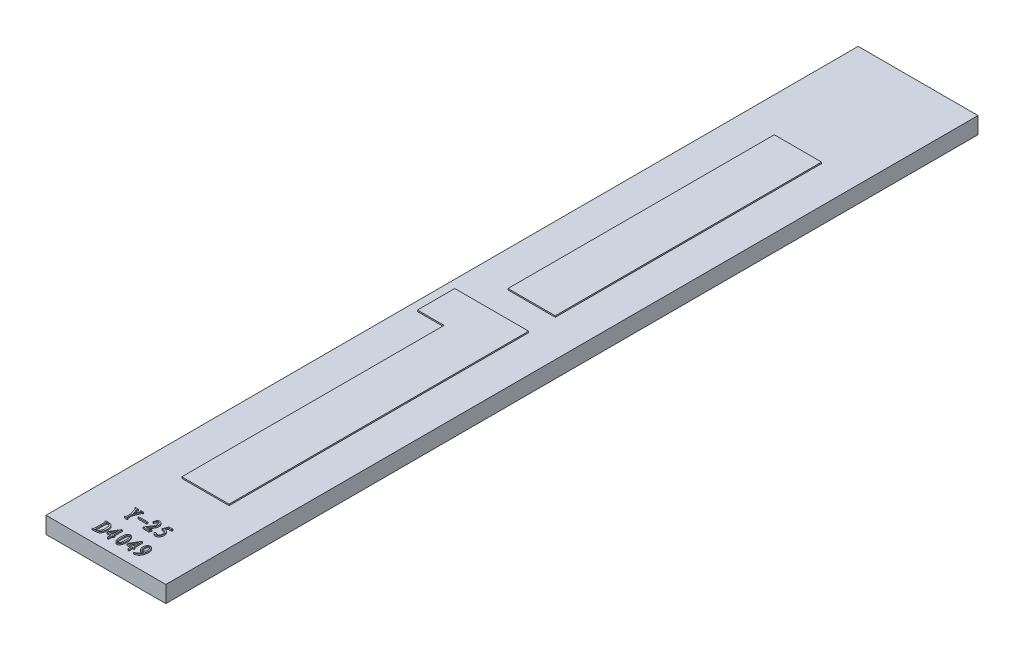
SolidWorks part; units mm, degrees
ref_plane "Front Plane" through (0, 0, 0) normal (0, 0, 1) x (1, 0, 0)
ref_plane "Top Plane" through (0, 0, 0) normal (0, 1, 0) x (1, 0, 0)
ref_plane "Right Plane" through (0, 0, 0) normal (1, 0, 0) x (0, 0, -1)
sketch "Sketch1" plane through (0, 0, 0) normal (0, 1, 0) x (1, 0, 0)
  line L1 (0, 0) -> (9, 0)
  line L2 (0, 0) -> (0, 61)
  line L3 (0, 61) -> (9, 61)
  line L4 (9, 0) -> (9, 61)
  dimension "D1" = 9
  dimension "D2" = 61
extrude "Boss-Extrude1" add sketch "Sketch1" along normal blind 1.25
sketch "Sketch2" plane through (0, 1.25, 0) normal (0, 1, 0) x (1, 0, 0)
  line L0 (0, 0) -> (9, 0) construction
  line L1 (2.7, 7.5) -> (6.25, 7.5)
  line L2 (2.7, 7.5) -> (2.7, 27.2)
  line L3 (0.7, 30) -> (6.25, 30)
  line L4 (6.25, 7.5) -> (6.25, 30)
  line L6 (2.7, 32) -> (6.25, 32)
  line L7 (2.7, 32) -> (2.7, 52)
  line L8 (2.7, 52) -> (6.25, 52)
  line L9 (6.25, 32) -> (6.25, 52)
  line L12 (2.7, 27.2) -> (0.7, 27.2)
  line L13 (0.7, 30) -> (0.7, 27.2)
  dimension "D1" = 7.5
  dimension "D2" = 3.55
  dimension "D3" = 22.5
  dimension "D4" = 20
  dimension "D5" = 2
  dimension "D6" = 2
  dimension "D7" = 2.8
extrude "Boss-Extrude2" add sketch "Sketch2" along normal blind 0.1
sketch "Sketch3" plane through (0, 1.25, 0) normal (0, 1, 0) x (1, 0, 0)
  line L0 (6.25, 32) -> (6.25, 52) construction
  line L1 (2.5, 34.0377) -> (2.5, 31.8)
  line L2 (6.45, 34.0377) -> (6.45, 31.8)
  line L3 (2.5, 31.8) -> (6.45, 31.8)
  line L4 (2.7, 52) -> (2.7, 32) construction
  line L5 (2.7, 32) -> (6.25, 32) construction
  line L6 (6.25, 30) -> (0.7, 30) construction
  line L7 (0.5, 30.2) -> (2.4897, 30.2)
  line L8 (0.5, 30.2) -> (0.5, 27)
  line L9 (0.5, 27) -> (2.4897, 27)
  line L10 (0.7, 27.2) -> (2.7, 27.2) construction
  line L11 (0.7, 30) -> (0.7, 27.2) construction
  point P8 (4.475, 32)
  dimension "D1" = 0.2
  dimension "D2" = 0.2
  dimension "D3" = 0.2
  dimension "D4" = 0.2
  dimension "D5" = 0.2
  dimension "D6" = 0.2
sketch "Sketch4" plane through (0, 1.25, 0) normal (0, 1, 0) x (1, 0, 0)
  text T0 "Y-25" font "Segoe UI" height 1
extrude "Boss-Extrude3" add sketch "Sketch4" along normal blind 0.1
sketch "Sketch6" plane through (0, 1.25, 0) normal (0, 1, 0) x (1, 0, 0)
  text T0 "D4049" font "Segoe UI" height 1
extrude "Boss-Extrude4" add sketch "Sketch6" along normal blind 0.1
